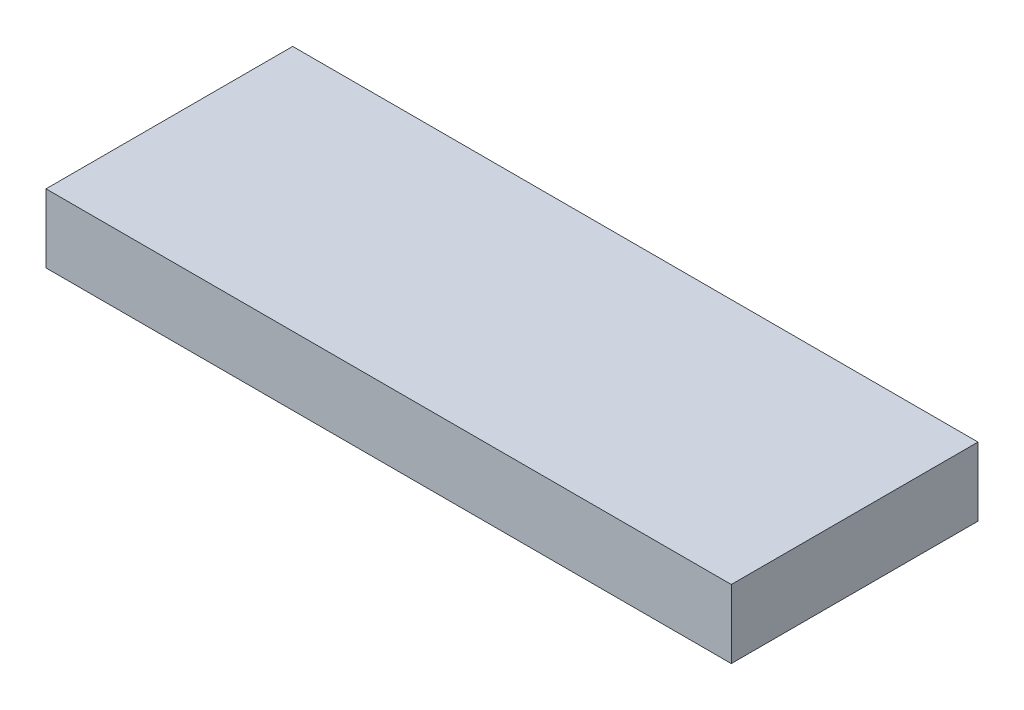
from build123d import *

# Parameters (mm, degrees)
SKETCH_1_W      = 500
SKETCH_1_H      = 180
EXTRUDE_1_DEPTH = 50


with BuildPart() as part:
    # 草图1 → 凸台-拉伸1 (new body)
    with BuildSketch(Plane(origin=(0, 0, 0), x_dir=(1, 0, 0), z_dir=(0, 1, 0))):
        Rectangle(SKETCH_1_W, SKETCH_1_H)
    extrude(amount=EXTRUDE_1_DEPTH)


solid = part.part
